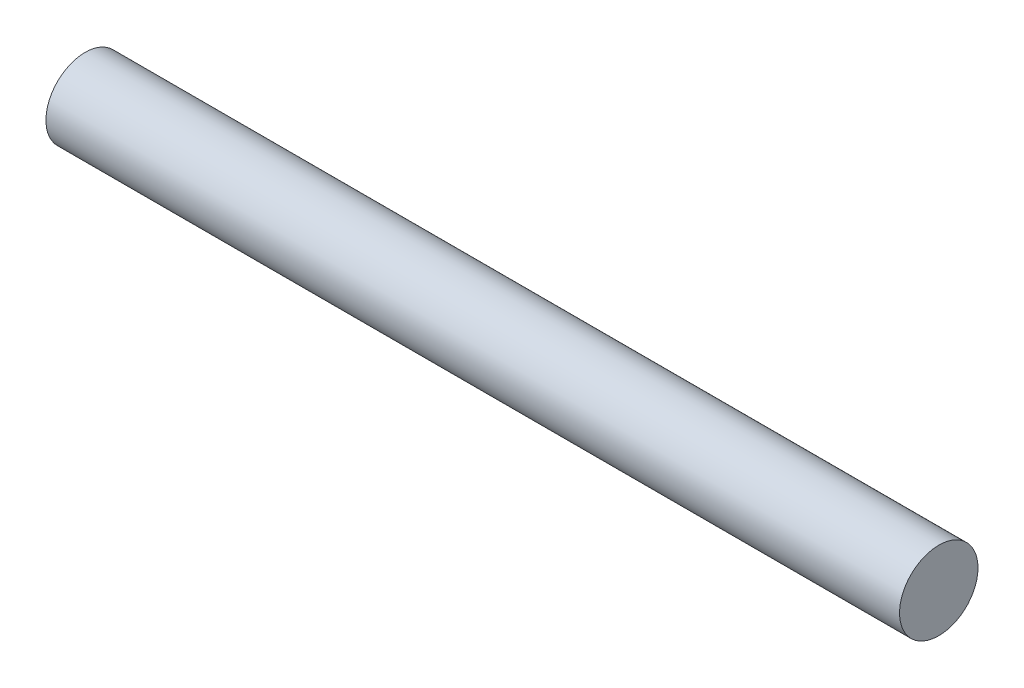
SolidWorks part; units mm, degrees
ref_plane "前视基准面" through (0, 0, 0) normal (0, 0, 1) x (1, 0, 0)
ref_plane "上视基准面" through (0, 0, 0) normal (0, 1, 0) x (1, 0, 0)
ref_plane "右视基准面" through (0, 0, 0) normal (1, 0, 0) x (0, 0, -1)
sketch "草图1" plane through (0, 0, 0) normal (1, 0, 0) x (0, 0, -1)
  circle A0 centre (0, 0) radius 12.5
  dimension "D1" = 25
extrude "凸台-拉伸1" add sketch "草图1" along normal mid plane 272
